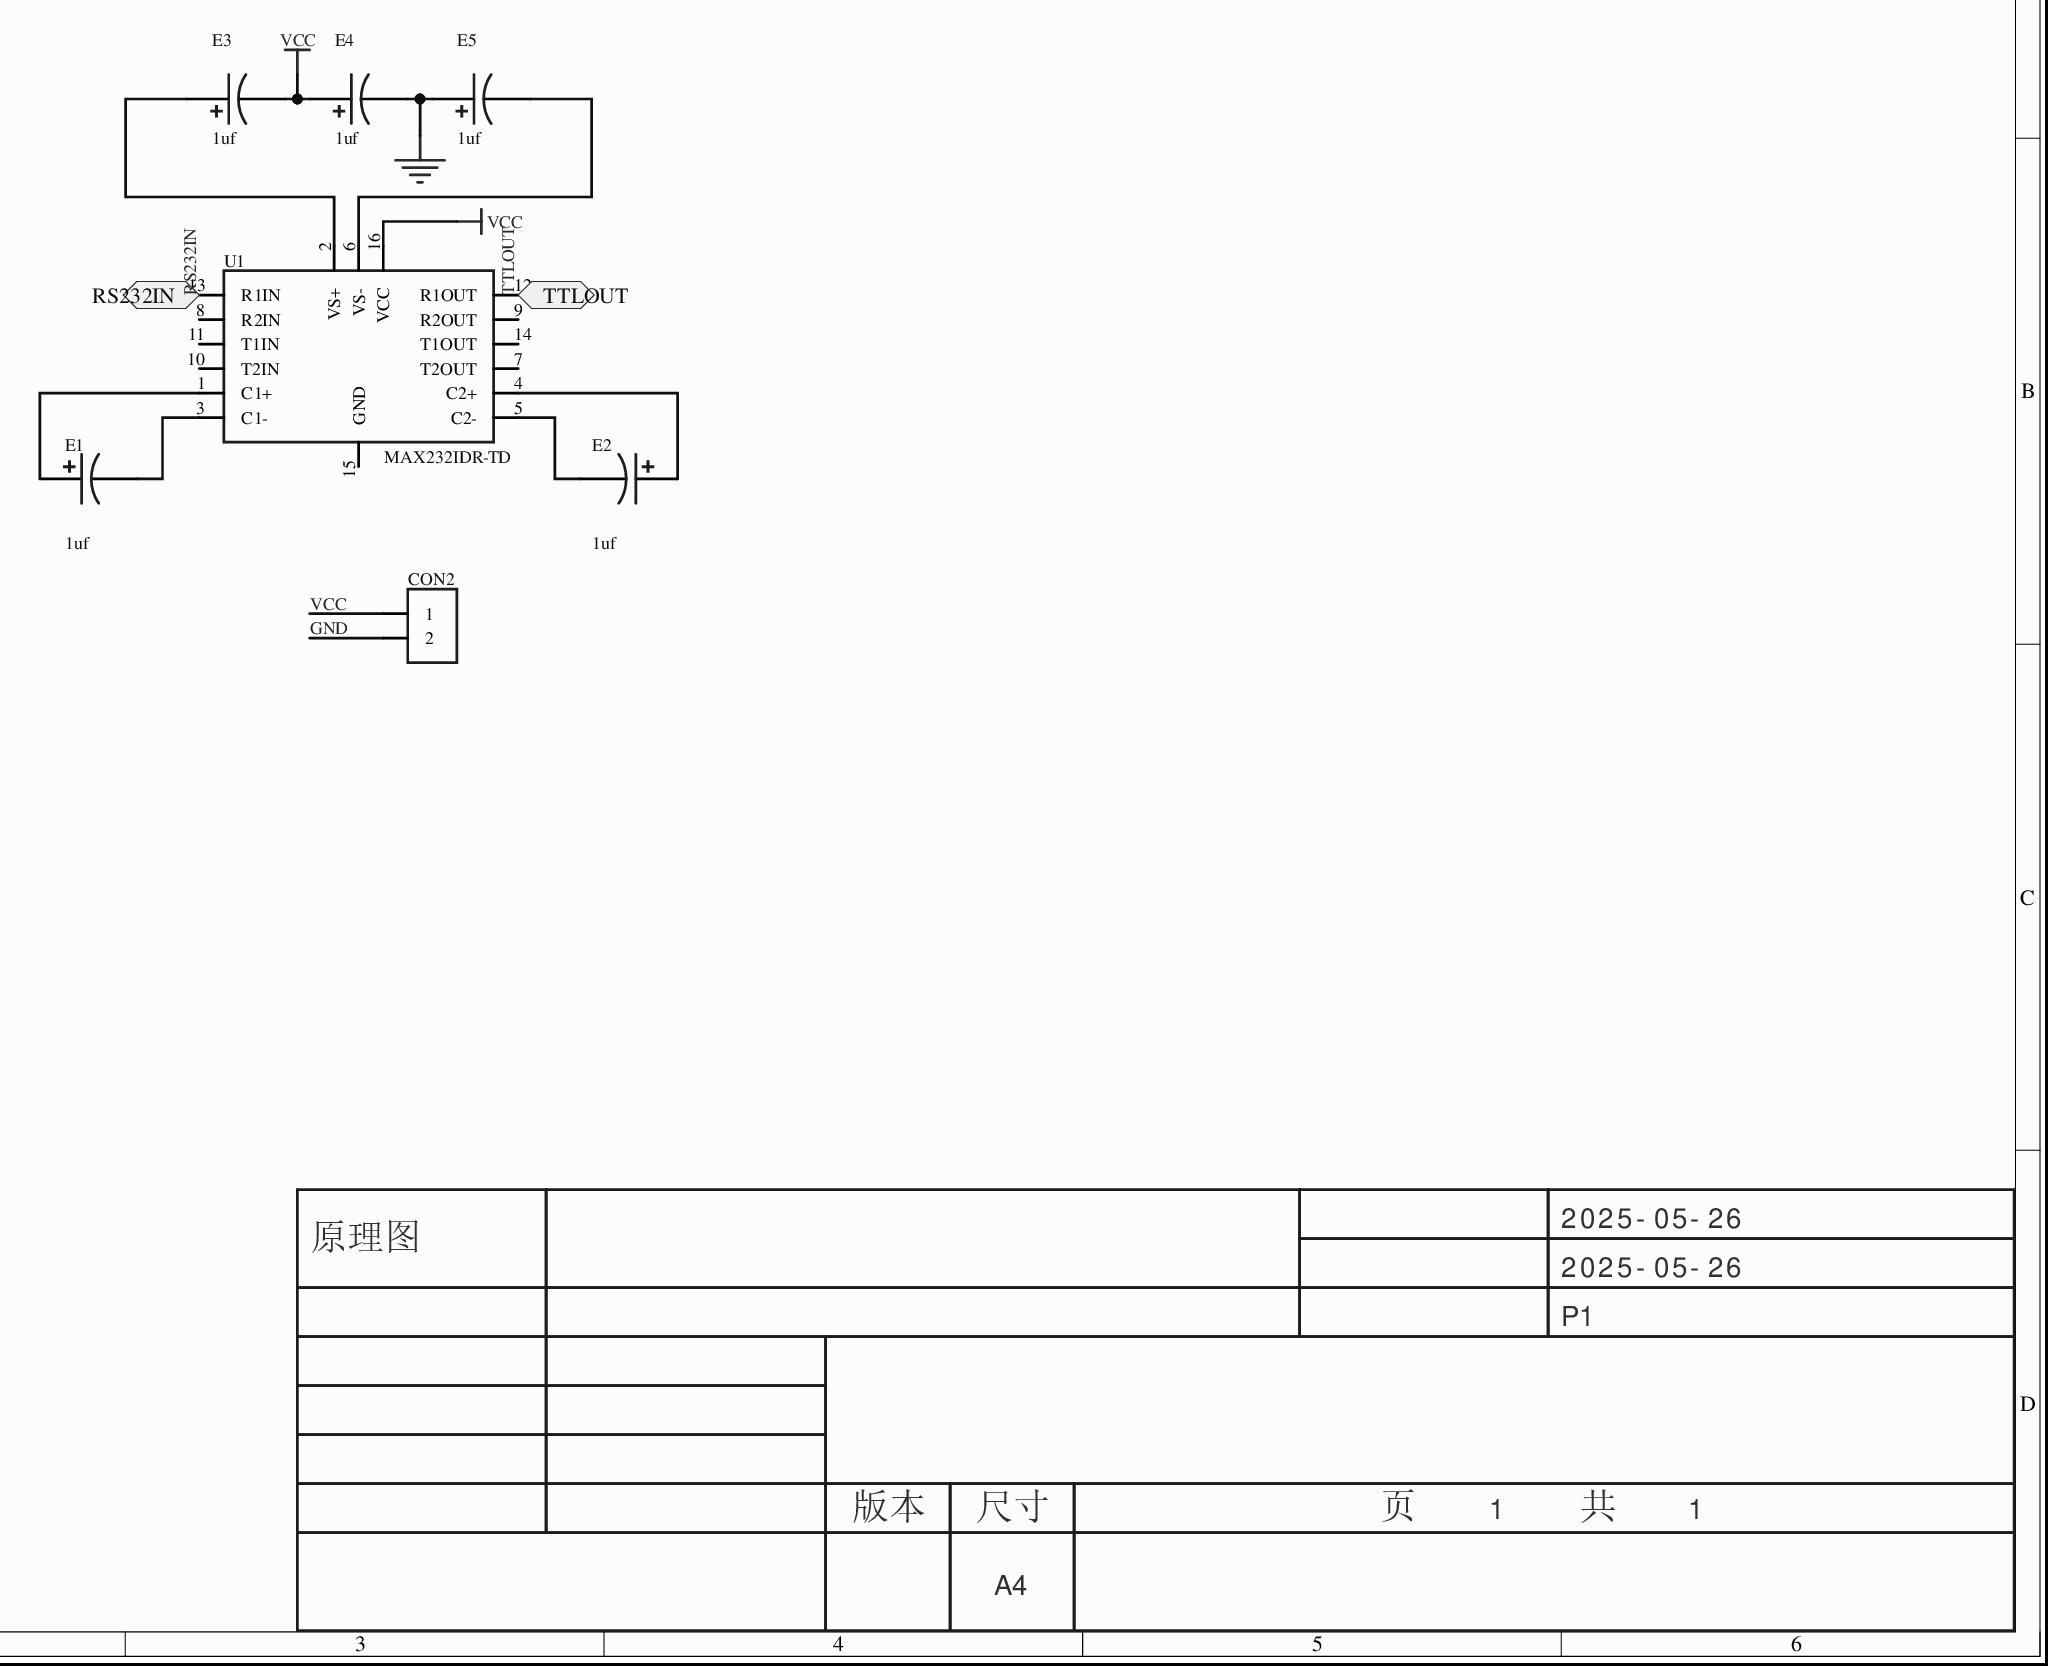
[diagram p0: MISC51987-3.schdoc]
# Altium project MISC51987-2.PrjPcb
1 sheet, 7 parts. Net scope: flat (ports and power ports of the same name join across sheets).
Board file: MISC51987.pcbdoc

## Sheet MISC51987-3.schdoc
size 297 x 209 mm; Version: V1.0; @Project Name: MISC51987; @Page Count: 1; @Update Date: 2025-05-26; @Create Date: 2025-05-26; @Schematic Name: MISC51987; @Page No: 1; @Create Time: 20:14:40; @Update Time: 20:35:44; @Board Name: MISC51987

### Parts
CON2  (no value)  [SIP-2_L2.0-W1.1-P0.90-D0.3]
E1  1uf  [CAP-TH_L17.0-W10.4-P5.08_CDK11A_470UF]
E2  1uf  [CAP-TH_L17.0-W10.4-P5.08_CDK11A_470UF]
E3  1uf  [CAP-TH_L17.0-W10.4-P5.08_CDK11A_470UF]
E4  1uf  [CAP-TH_L17.0-W10.4-P5.08_CDK11A_470UF]
E5  1uf  [CAP-TH_L17.0-W10.4-P5.08_CDK11A_470UF]
U1  MAX232IDR-TD  [DIP-16_L19.7-W6.6-P2.54-LS10.9-BL]

### Ports
RS232IN (bidir), TTLOUT (bidir)

### Nets
GND: CON2.2 E4.2 E5.1
VCC: CON2.1 E3.2 E4.1 U1.16(VCC)
RS232IN: U1.13(R1IN) ; port RS232IN
TTLOUT: U1.12(R1OUT) ; port TTLOUT
NetE1_1: E1.1 U1.1(C1+)
NetE1_2: E1.2 U1.3(C1-)
NetE2_1: E2.1 U1.4(C2+)
NetE2_2: E2.2 U1.5(C2-)
NetE3_1: E3.1 U1.2(VS+)
NetE5_2: E5.2 U1.6(VS-)

Not connected (* = marked no-connect by the designer): U1 7(T2OUT) 8(R2IN) 9(R2OUT) 10(T2IN) 11(T1IN) 14(T1OUT) 15(GND)

### Notes on the sheet
- 2025-05-26
- 原理图
- P1
- 版本
- 尺寸
- A4
- 页    1    共    1

### Library data of the parts
CON2 = HDR-F_2.54_1x2P: Symbol: Header-Female-2.54_1x2; ConvertToPcb: yes; ModelId: a9450ef445564560a104363b9aacde4e; ModelName: HDR-TH_2P-P2.54-F-LI-1X2P; ModelTransform: 215.7476,98.425,0,0,0,0,0,0,-129.921; Device: HDR-F_2.54_1x2P; AddInBom: yes; SupplierPart: C49661; Supplier Footprint: 插件; FootprintName: SIP-2_L2.0-W1.1-P0.90-D0.3
E1-E5 = 10uf: Symbol: 10UF_C9900016685; AddInBom: yes; ModelId: 1f26856de1634853a779dc49a005d0a1; ModelName: CAP-SMD_L2.0-W1.3-FD; ModelTransform: 78.74,49.2125,0,0,0,0,0,-0.551,0; Manufacturer Part: 1uf; Device: 10uf; LCSC Part Name: 10uf; SupplierPart: C9900016685; Supplier Footprint: SMD,2x1.25x1.2mm; JLCPCB Part Class: 扩展库; Supplier: LCSC; ConvertToPcb: yes; FootprintName: CAP-TH_L17.0-W10.4-P5.08_CDK11A_470UF
U1 = MAX232IDR-TD: 类型:收发器;数据速率:120Kbps;; Manufacturer: TDSEMIC(拓电半导体); AddInBom: yes; Number of Drivers: 2; Voltage - Supply: 4.5V~5.5V; charge pump: 有; ModelId: c21ec766ec2643efb3352f8441994f4e; ModelName: SOIC-16_L9.9-W3.9-H1.8-LS6.0-P1.27; ModelTransform: 389.763,236.454,0,0,0,0,0,0,0; Symbol: MAX232IDR-TD; Device: MAX232IDR-TD; LCSC Part Name: MAX232IDR-TD; SupplierPart: C42422010; ManufacturerPart: MAX232IDR-TD; Supplier Footprint: SOP-16; Datasheet: https://atta.szlcsc.com/upload/public/pdf/source/20241227/DBBA0EE2A2E10E2AC0CAF98D845AFDAB.pdf; Supplier: LCSC; ConvertToPcb: yes; Type: 收发器; Number of Receivers: 2; Data Rate: 120Kbps; FootprintName: DIP-16_L19.7-W6.6-P2.54-LS10.9-BL